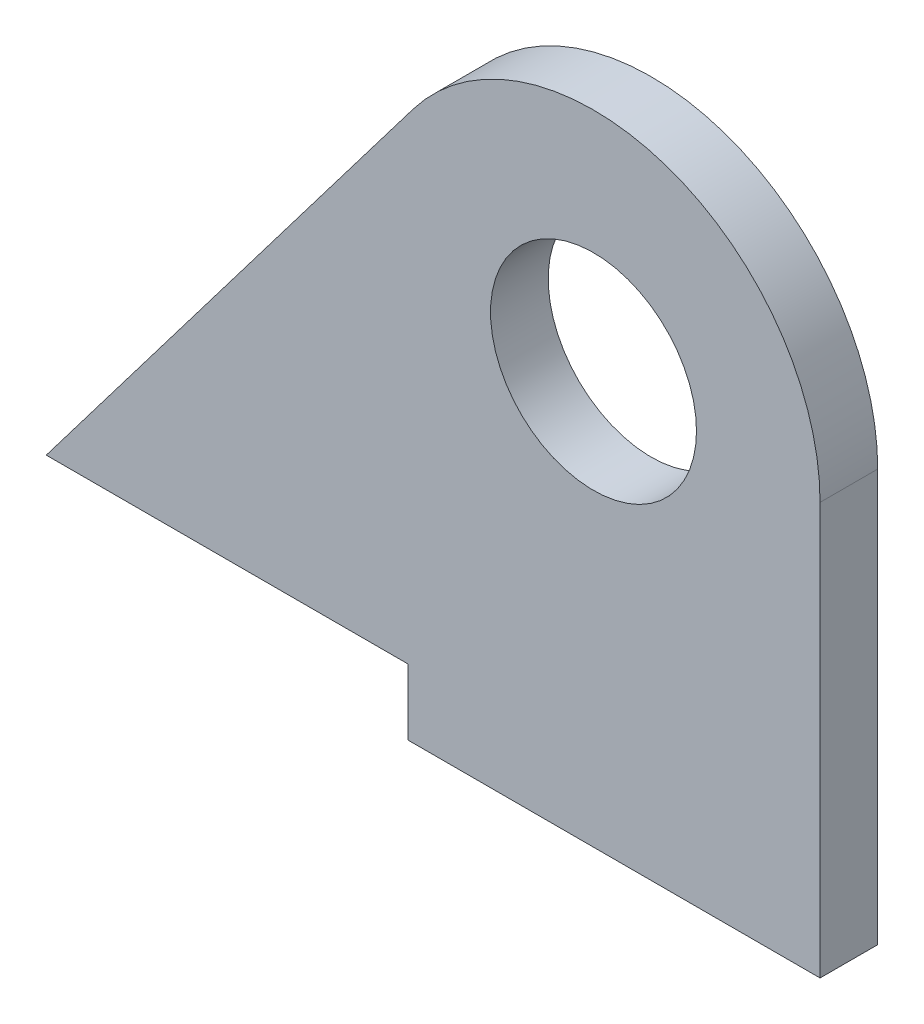
from build123d import *

# Parameters (mm, degrees)
SKETCH1_R           = 25
BOSS_EXTRUDE1_DEPTH = 14
SKETCH2_W           = 100
SKETCH2_H           = 16
CUT_EXTRUDE1_DEPTH  = 177.694651872


with BuildPart() as part:
    # Sketch1 → Boss-Extrude1 (new body)
    with BuildSketch(Plane.XY):
        with BuildLine():
            Line((-43.801805937, 33.262618608), (-145, -100))
            Line((-145, -100), (55, -100))
            Line((55, -100), (55, 0))
            ThreePointArc((55, 0), (17.548513804, 52.125326505), (-43.801805937, 33.262618608))
        make_face()
        Circle(SKETCH1_R, mode=Mode.SUBTRACT)
    extrude(amount=BOSS_EXTRUDE1_DEPTH)

    # Sketch2 → Cut-Extrude1 (cut, through all)
    with BuildSketch(Plane.XY.offset(14)):
        with Locations((-95, -92)):
            Rectangle(SKETCH2_W, SKETCH2_H)
    extrude(amount=-CUT_EXTRUDE1_DEPTH, mode=Mode.SUBTRACT)


solid = part.part
